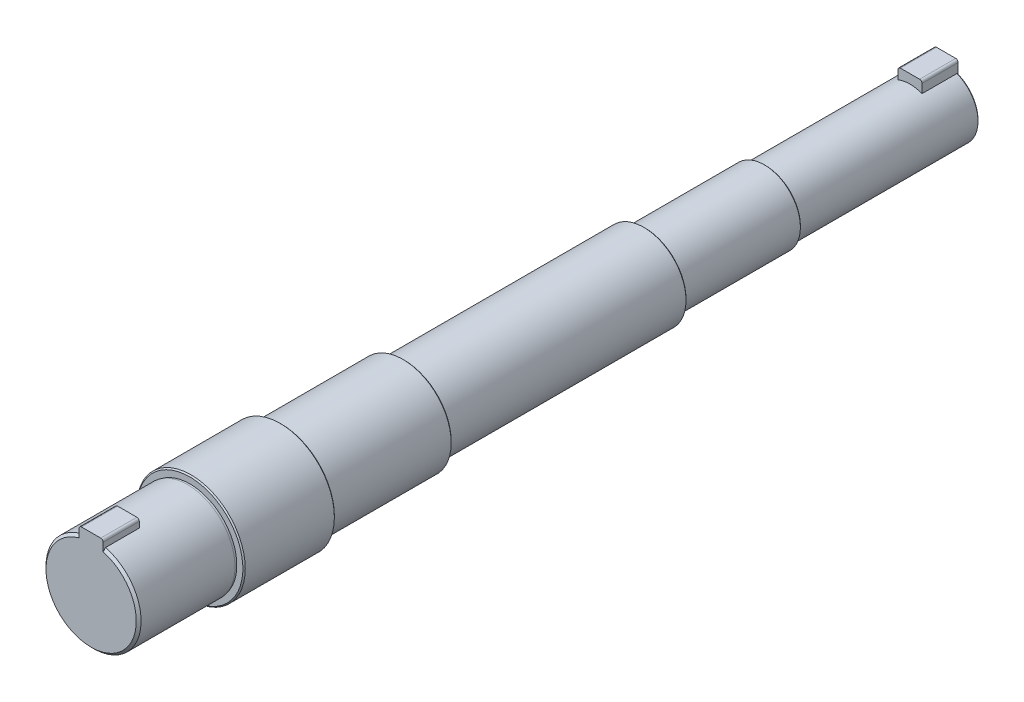
SolidWorks part; units mm, degrees
ref_plane "Front Plane" through (0, 0, 0) normal (0, 0, 1) x (1, 0, 0)
ref_plane "Top Plane" through (0, 0, 0) normal (0, 1, 0) x (1, 0, 0)
ref_plane "Right Plane" through (0, 0, 0) normal (1, 0, 0) x (0, 0, -1)
other "Configuration Table"
sketch "Sketch1" plane through (0, 0, 0) normal (0, 0, 1) x (1, 0, 0)
  circle A0 centre (0, 0) radius 3.95
  dimension "D1" = 7.9
extrude "Boss-Extrude1" add sketch "Sketch1" along normal blind 8 contours A0
ref_plane "Plane1" through (0, 0, 5) normal (0, 0, -1) x (-1, 0, 0)
sketch "Sketch2" plane through (0, 0, 5) normal (0, 0, -1) x (-1, 0, 0)
  line L1 (-1, 4.5) -> (1, 4.5)
  line L2 (-1, 4.5) -> (-1, 3)
  line L3 (-1, 3) -> (1, 3)
  line L4 (1, 4.5) -> (1, 3)
  point P4 (0, 3)
  dimension "D1" = 4.5
  dimension "D2" = 3
  dimension "D3" = 2
extrude "Boss-Extrude2" add sketch "Sketch2" against normal up to surface (3 mm away) up to face at (3.95, 0, 8)
fillet "Fillet1" radius 0.2 2 edges at (1, 4.5, 6.5) (-1, 4.5, 6.5)
sketch "Sketch3" plane through (0, 0, 0) normal (0, 0, -1) x (-1, 0, 0)
  circle A0 centre (0, 0) radius 3.9
  dimension "D1" = 7.8
extrude "Boss-Extrude3" add sketch "Sketch3" along normal blind 0.2 contours A0
sketch "Sketch4" plane through (0, 0, -0.2) normal (0, 0, -1) x (-1, 0, 0)
  circle A0 centre (0, 0) radius 4.5
  dimension "D1" = 9
extrude "Boss-Extrude4" add sketch "Sketch4" along normal blind 7.6 contours A0
sketch "Sketch6" plane through (0, 0, -7.8) normal (0, 0, -1) x (-1, 0, 0)
  circle A0 centre (0, 0) radius 3.9 construction
  circle A1 centre (0, 0) radius 3.9
extrude "Boss-Extrude5" add sketch "Sketch6" along normal blind 0.2 contours A1
sketch "Sketch7" plane through (0, 0, -8) normal (0, 0, -1) x (-1, 0, 0)
  circle A2 centre (0, 0) radius 4
  dimension "D1" = 8
chamfer "Chamfer2" distance 0.2 angle 45 1 edges at (0, -3.95, 8)
extrude "Boss-Extrude8" add sketch "Sketch7" along normal blind 10 contours A2
sketch "Sketch9" plane through (0, 0, -18) normal (0, 0, -1) x (-1, 0, 0)
  circle A0 centre (0, 0) radius 3.5
  dimension "D1" = 7
extrude "Boss-Extrude9" add sketch "Sketch9" along normal blind 20 contours A0
sketch "Sketch10" plane through (0, 0, -38) normal (0, 0, -1) x (-1, 0, 0)
  circle A0 centre (0, 0) radius 3
  dimension "D1" = 6
extrude "Boss-Extrude10" add sketch "Sketch10" along normal blind 10 contours A0
ref_plane "Plane2" through (0, 0, -68) normal (0, 0, -1) x (-1, 0, 0)
sketch "Sketch12" plane through (0, 0, -68) normal (0, 0, -1) x (-1, 0, 0)
sketch "Sketch13" plane through (0, 0, -48) normal (0, 0, -1) x (-1, 0, 0)
  circle A0 centre (0, 0) radius 2.75
  dimension "D1" = 5.5
extrude "Boss-Extrude11" add sketch "Sketch13" along normal blind 15 contours A0
ref_plane "Plane3" through (0, 0, -60) normal (0, 0, -1) x (-1, 0, 0)
sketch "Sketch14" plane through (0, 0, -60) normal (0, 0, -1) x (-1, 0, 0)
  line L1 (-1, 3.5) -> (1, 3.5)
  line L2 (-1, 3.5) -> (-1, 2.5617)
  line L4 (1, 3.5) -> (1, 2.5617)
  circle A1 centre (0, 0) radius 2.75
  arc A2 (1, 2.5617) -> (-1, 2.5617) centre (0, 0) ccw
  dimension "D2" = 2
  dimension "D3" = 3.5
  dimension "D4" = 1
  dimension "D1" = 0
extrude "Boss-Extrude13" add sketch "Sketch14" along normal up to surface (3 mm away) contours L1 L4 A2 L2 up to face at (-2.75, 0, -63)
fillet "Fillet2" radius 0.2 2 edges at (-1, 3.5, -61.5) (1, 3.5, -61.5)
chamfer "Chamfer5" distance 0.1 angle 45 6 edges at (-4.5, 0, -0.2) (-4.5, 0, -7.8) (-4, 0, -18) (-3.5, 0, -38) (-3, 0, -48) (0, -2.75, -63)
